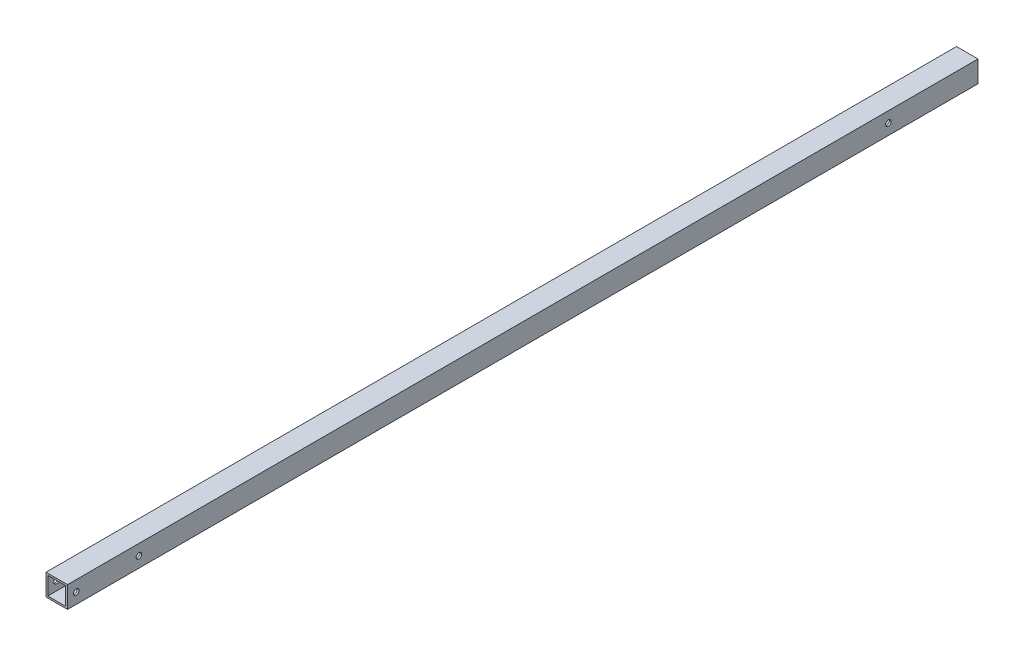
from build123d import *

# Parameters (mm, degrees)
SKETCH_1_W               = 12
SKETCH_1_H               = 12
SKETCH_1_W_2             = 10
SKETCH_1_H_2             = 10
EXTRUDE_1_DEPTH          = 516
CUT_EXTRUDE_1_DEPTH      = 517.174389136
CUT_EXTRUDE_1_DEPTH_BACK = 517.174389136
SKETCH_2_R               = 1.55
SKETCH_3_W               = 12
SKETCH_3_H               = 12
SKETCH_3_W_2             = 10
SKETCH_3_H_2             = 10
CUT_EXTRUDE_2_DEPTH      = 8


with BuildPart() as part:
    # 草图1 → 凸台-拉伸1 (new body)
    with BuildSketch(Plane.XY):
        Rectangle(SKETCH_1_W, SKETCH_1_H)
        Rectangle(SKETCH_1_W_2, SKETCH_1_H_2, mode=Mode.SUBTRACT)
    extrude(amount=EXTRUDE_1_DEPTH)

    # 草图2 → 切除-拉伸1 (cut, two sides: drawn at the far end of the back side and taken through both)
    with BuildSketch(Plane.ZY.offset(6).offset(-CUT_EXTRUDE_1_DEPTH_BACK)):
        with Locations(Location((50, 0, 0), (0, 0, 180))):
            Circle(SKETCH_2_R)
        with Locations(Location((468.132973417, 0, 0), (0, 0, 180))):
            Circle(SKETCH_2_R)
        with Locations(Location((503.132973417, 0, 0), (0, 0, 180))):
            Circle(SKETCH_2_R)
    extrude(amount=CUT_EXTRUDE_1_DEPTH + CUT_EXTRUDE_1_DEPTH_BACK, mode=Mode.SUBTRACT)

    # 草图3 → 切除-拉伸2 (cut)
    with BuildSketch(Plane.XY.offset(516)):
        Rectangle(SKETCH_3_W, SKETCH_3_H)
        Rectangle(SKETCH_3_W_2, SKETCH_3_H_2, mode=Mode.SUBTRACT)
    extrude(amount=-CUT_EXTRUDE_2_DEPTH, mode=Mode.SUBTRACT)


solid = part.part
